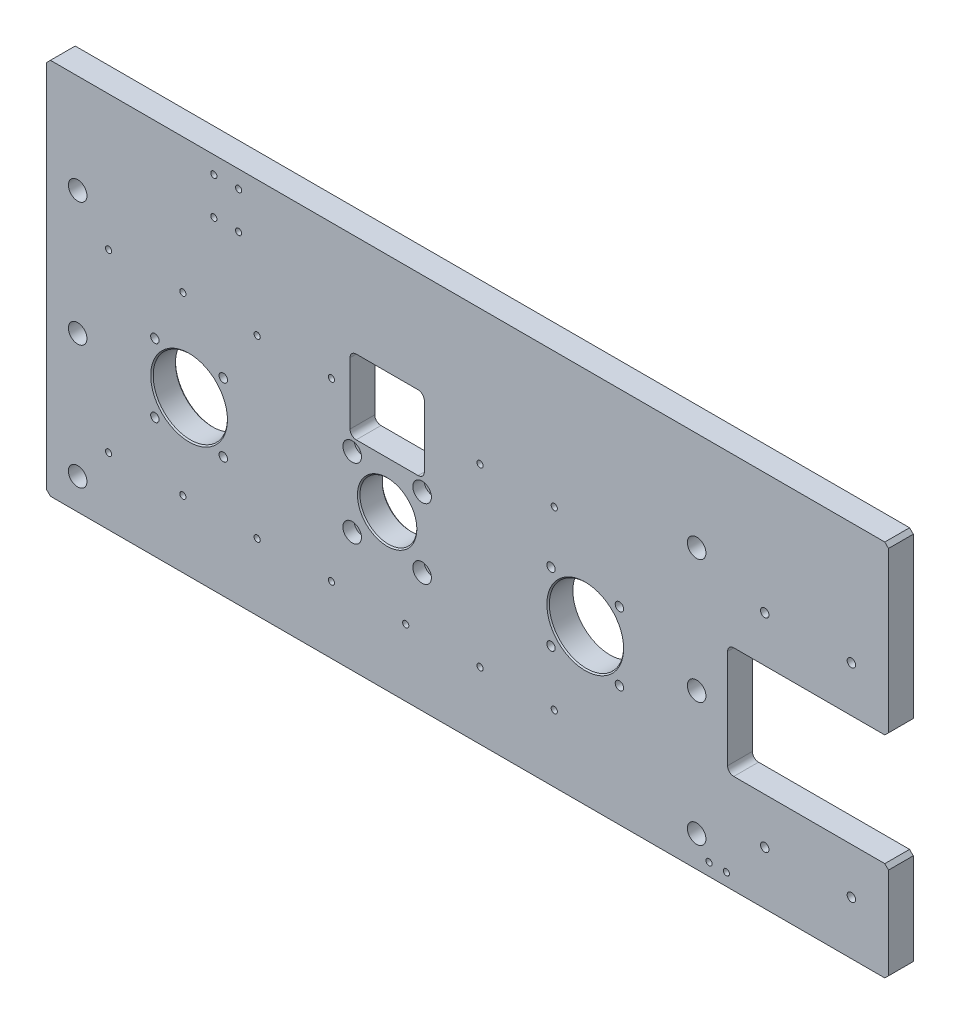
from build123d import *

# Parameters (mm, degrees)
SKETCH1_W             = 60
SKETCH1_H             = 60
BOSS_EXTRUDE1_DEPTH   = 20
FILLET1_R             = 5
CHAMFER1_SIZE         = 3
SKETCH2_R             = 30
SKETCH2_R_2           = 23
CUT_EXTRUDE1_DEPTH    = 20
CHAMFER2_SIZE         = 1
M8_TAPPED_HOLE1_D     = 6.8
M6_TAPPED_HOLE1_D     = 5
M6_TAPPED_HOLE2_D     = 5
M6_TAPPED_HOLE2_DEPTH = 13
M6_TAPPED_HOLE2_TIP   = 1.502151548
M8_TAPPED_HOLE2_D     = 6.8
M6_TAPPED_HOLE3_D     = 5
HOLE1_D               = 9
HOLE1_CBORE_D         = 15
HOLE1_CBORE_DEPTH     = 11
HOLE2_D               = 9
HOLE2_CBORE_D         = 15
HOLE2_CBORE_DEPTH     = 9


with BuildPart() as part:
    # Sketch1 → Boss-Extrude1 (new body)
    with BuildSketch(Plane.XY):
        Polygon((421.759394592, -47.943047911), (421.759394592, -127.943047911), (-258.240605408, -127.943047911), (-258.240605408, 177.056952089), (421.759394592, 177.056952089), (421.759394592, 42.056952089), (291.759394592, 42.056952089), (291.759394592, -47.943047911), align=None)
        with Locations((16.759394592, 65.056952089)):
            Rectangle(SKETCH1_W, SKETCH1_H, mode=Mode.SUBTRACT)
    extrude(amount=BOSS_EXTRUDE1_DEPTH)

    # Fillet1
    fillet1_edges = [part.edges().sort_by_distance(p)[0] for p in [
        (291.759394592, 42.056952089, 10),
        (291.759394592, -47.943047911, 10),
        (-13.240605408, 95.056952089, 10),
        (-13.240605408, 35.056952089, 10),
        (46.759394592, 35.056952089, 10),
        (46.759394592, 95.056952089, 10),
    ]]
    fillet(fillet1_edges, radius=FILLET1_R)

    # Chamfer1
    chamfer1_edges = [part.edges().sort_by_distance(p)[0] for p in [
        (-258.240605408, 177.056952089, 10),
        (421.759394592, 177.056952089, 10),
        (421.759394592, 42.056952089, 10),
        (421.759394592, -47.943047911, 10),
        (421.759394592, -127.943047911, 10),
        (-258.240605408, -127.943047911, 10),
    ]]
    chamfer(chamfer1_edges, length=CHAMFER1_SIZE)

    # Sketch2 → Cut-Extrude1 (cut)
    with BuildSketch(Plane.XY.offset(20)):
        with Locations((-143.240605408, -2.943047911)):
            Circle(SKETCH2_R)
        with Locations((16.759394592, -2.943047911)):
            Circle(SKETCH2_R_2)
        with Locations((176.759394592, -2.943047911)):
            Circle(SKETCH2_R)
    extrude(amount=-CUT_EXTRUDE1_DEPTH, mode=Mode.SUBTRACT)

    # Chamfer2
    chamfer2_edges = [part.edges().sort_by_distance(p)[0] for p in [
        (-173.240605408, -2.943047911, 0),
        (-173.240605408, -2.943047911, 20),
        (-6.240605408, -2.943047911, 0),
        (-6.240605408, -2.943047911, 20),
        (146.759394592, -2.943047911, 20),
    ]]
    chamfer(chamfer2_edges, length=CHAMFER2_SIZE)

    # M8 Tapped Hole1 (through all)
    with Locations(Plane.XY.offset(20)):
        with Locations((321.759394592, 79.056952089), (391.759394592, 79.056952089), (391.759394592, -84.943047911), (321.759394592, -84.943047911)):
            Hole(M8_TAPPED_HOLE1_D / 2)

    # M6 Tapped Hole1 (through all)
    with Locations(Plane.XY.offset(20)):
        with Locations((276.759394592, -117.943047911), (290.759394592, -117.943047911)):
            Hole(M6_TAPPED_HOLE1_D / 2)

    # M6 Tapped Hole2
    with Locations(Plane.XY.offset(20)):
        with Locations((-208.240605408, 68.056952089), (-208.240605408, -73.943047911), (-148.240605408, -73.943047911), (-88.240605408, -73.943047911), (-88.240605408, 68.056952089), (-148.240605408, 68.056952089), (-28.240605408, 68.056952089), (-28.240605408, -73.943047911), (31.759394592, -73.943047911), (91.759394592, -73.943047911), (151.759394592, -73.943047911), (151.759394592, 68.056952089), (91.759394592, 68.056952089)):
            Hole(M6_TAPPED_HOLE2_D / 2, depth=M6_TAPPED_HOLE2_DEPTH)
            with Locations((0, 0, -(M6_TAPPED_HOLE2_DEPTH + M6_TAPPED_HOLE2_TIP / 2))):  # 118° drill point
                Cone(0, M6_TAPPED_HOLE2_D / 2, M6_TAPPED_HOLE2_TIP, mode=Mode.SUBTRACT)

    # M8 Tapped Hole2 (through all)
    with Locations(Plane.XY.offset(20)):
        with Locations((-170.871260926, 24.687607606), (-170.871260926, -30.573703429), (-115.609949891, -30.573703429), (-115.609949891, 24.687607606), (149.128739074, 24.687607606), (204.390050109, 24.687607606), (204.390050109, -30.573703429), (149.128739074, -30.573703429)):
            Hole(M8_TAPPED_HOLE2_D / 2)

    # M6 Tapped Hole3 (through all)
    with Locations(Plane.XY.offset(20)):
        with Locations((-123.240605408, 163.056952089), (-103.240605408, 163.056952089), (-103.240605408, 133.056952089), (-123.240605408, 133.056952089)):
            Hole(M6_TAPPED_HOLE3_D / 2)

    # Hole1 (through all)
    with Locations(Plane.XY.offset(20)):
        with Locations((-233.240605408, 97.056952089), (-233.240605408, -2.943047911), (-233.240605408, -102.943047911), (266.759394592, 97.056952089), (266.759394592, -102.943047911), (266.759394592, -2.943047911)):
            CounterBoreHole(HOLE1_D / 2, HOLE1_CBORE_D / 2, HOLE1_CBORE_DEPTH)

    # Hole2 (through all)
    with Locations(Plane.XY.offset(20)):
        with Locations((-11.490605408, 25.306952089), (45.009394592, 25.306952089), (45.009394592, -31.193047911), (-11.490605408, -31.193047911)):
            CounterBoreHole(HOLE2_D / 2, HOLE2_CBORE_D / 2, HOLE2_CBORE_DEPTH)


solid = part.part
